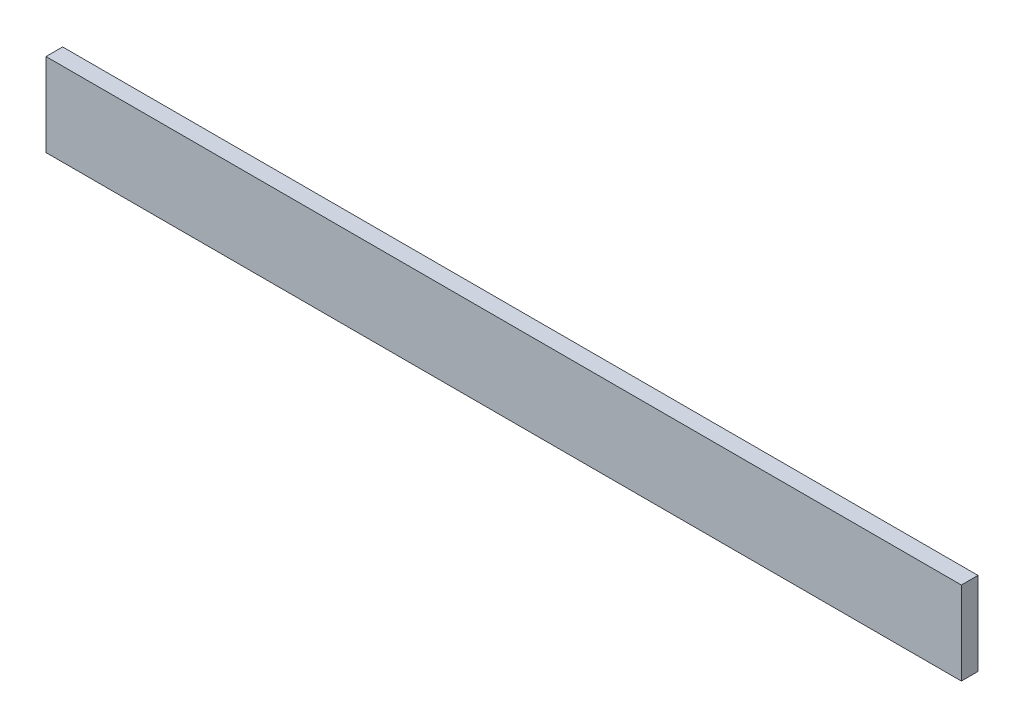
SolidWorks part; units mm, degrees
ref_plane "Front Plane" through (0, 0, 0) normal (0, 0, 1) x (1, 0, 0)
ref_plane "Top Plane" through (0, 0, 0) normal (0, 1, 0) x (1, 0, 0)
ref_plane "Right Plane" through (0, 0, 0) normal (1, 0, 0) x (0, 0, -1)
other "Configuration Table"
sketch "Sketch1" plane through (0, 0, 0) normal (0, 0, 1) x (1, 0, 0)
  line L13 (0, 0) -> (1100, 0)
  line L14 (0, 0) -> (0, 100)
  line L15 (0, 100) -> (1100, 100)
  line L16 (1100, 0) -> (1100, 100)
  dimension "D1" = 1100
  dimension "D2" = 100
extrude "Boss-Extrude1" add sketch "Sketch1" along normal blind 20
